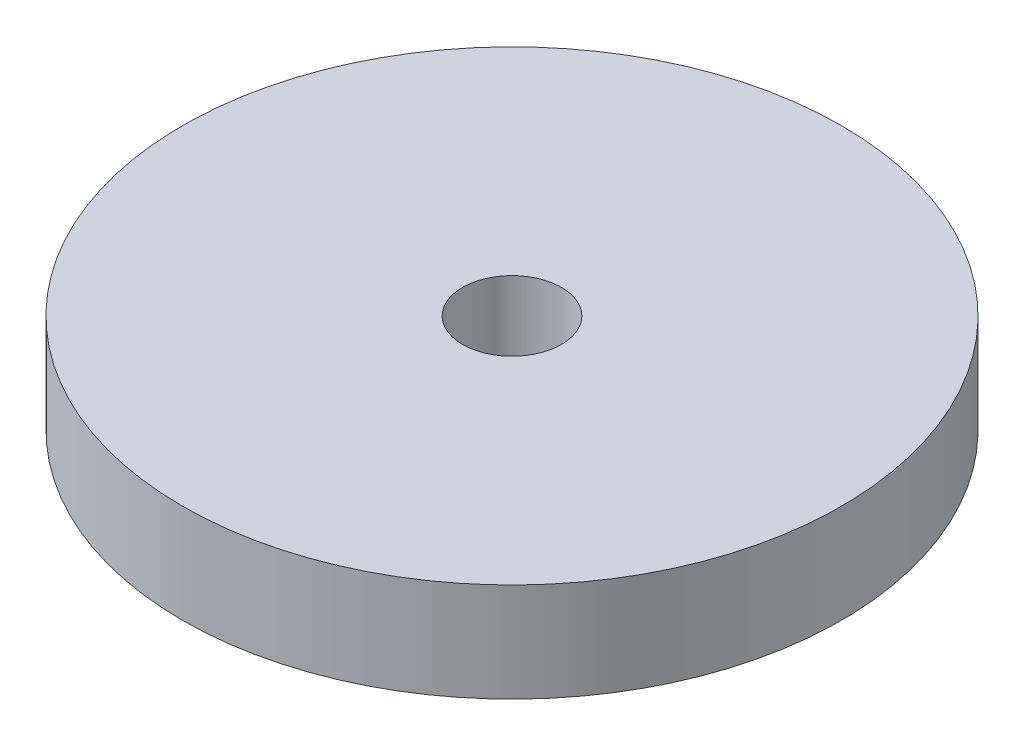
SolidWorks part; units mm, degrees
ref_plane "前视基准面" through (0, 0, 0) normal (0, 0, 1) x (1, 0, 0)
ref_plane "上视基准面" through (0, 0, 0) normal (0, 1, 0) x (1, 0, 0)
ref_plane "右视基准面" through (0, 0, 0) normal (1, 0, 0) x (0, 0, -1)
sketch "草图1" plane through (0, 0, 0) normal (1, 0, 0) x (0, 0, -1)
  line L0 (0, 36.72) -> (0, -20.91) construction
  line L1 (15, 0) -> (100, 0)
  line L2 (100, 30) -> (15, 30)
  line L4 (100, 30) -> (100, 0)
  line L5 (15, 30) -> (15, 0)
  dimension "D1" = 100
  dimension "D2" = 15
revolve "旋转2" add sketch "草图1" angle 360 about L0
